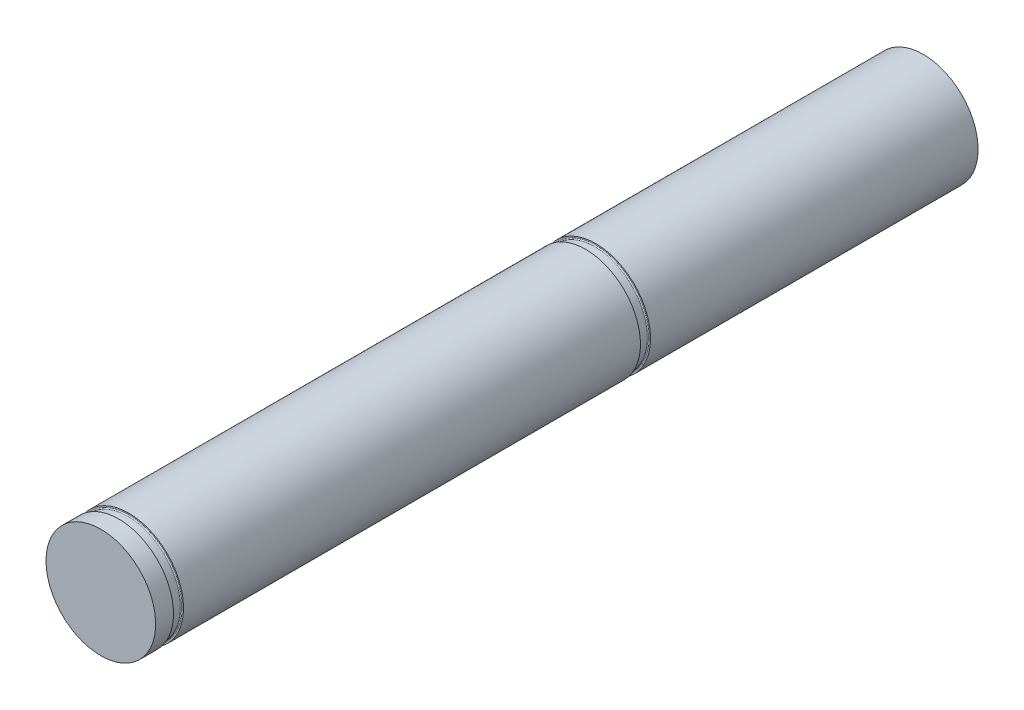
from build123d import *

# Parameters (mm, degrees)
SKETCH_1_R             = 6
EXTRUDE_1_DEPTH        = 90
PATTERN_LINEAR_1_COUNT = 2
PATTERN_LINEAR_1_PITCH = 51.1
HOLE_WIZARD_M6_1_D     = 5
HOLE_WIZARD_M6_1_DEPTH = 11
HOLE_WIZARD_M6_1_TIP   = 1.502151548


with BuildPart() as part:
    # 草图1 → 凸台-拉伸1 (new body)
    with BuildSketch(Plane.XY):
        with Locations(Location((0, 0, 0), (0, 0, 180))):
            Circle(SKETCH_1_R)
    extrude(amount=EXTRUDE_1_DEPTH)

    # Groove Sketch → Retaining Ring Groove (revolve, cut)
    with BuildSketch(Plane(origin=(4.683915956, 3.689622128, 8.399116992), x_dir=(-0.5195228612321346, -0.40923941910457057, 0.7500793921366791), z_dir=(0.6187960743401806, -0.785551664998033, 0)), mode=Mode.PRIVATE) as retaining_ring_groove_sk:
        with BuildLine():
            Line((67.563324222, -43.809060949), (67.655912914, -43.704049834))
            Line((67.655912914, -43.704049834), (66.830825582, -42.97656726))
            Line((66.830825582, -42.97656726), (66.738236891, -43.081578375))
            ThreePointArc((66.738236891, -43.081578375), (66.710962353, -43.161228331), (66.747997367, -43.236835366))
            Line((66.747997367, -43.236835366), (67.408067232, -43.818821425))
            ThreePointArc((67.408067232, -43.818821425), (67.487717188, -43.846095963), (67.563324222, -43.809060949))
        make_face()
    retaining_ring_groove = revolve(retaining_ring_groove_sk.sketch.rotate(Axis((0, 0, 41.519998945), (0, 0, -1)), 128.228270648), axis=Axis((0, 0, 41.519998945), (0, 0, -1)), mode=Mode.SUBTRACT)

    # 阵列(线性)1: Retaining Ring Groove ×2
    with Locations(*[(0, 0, -i * PATTERN_LINEAR_1_PITCH) for i in range(1, PATTERN_LINEAR_1_COUNT)]):
        add(retaining_ring_groove, mode=Mode.SUBTRACT)

    # M6 螺纹孔1
    with Locations(Plane(origin=(0, 0, 0), x_dir=(-1, 0, 0), z_dir=(0, 0, -1))):
        with Locations((0, 0)):
            Hole(HOLE_WIZARD_M6_1_D / 2, depth=HOLE_WIZARD_M6_1_DEPTH)
            with Locations((0, 0, -(HOLE_WIZARD_M6_1_DEPTH + HOLE_WIZARD_M6_1_TIP / 2))):  # 118° drill point
                Cone(0, HOLE_WIZARD_M6_1_D / 2, HOLE_WIZARD_M6_1_TIP, mode=Mode.SUBTRACT)


solid = part.part
